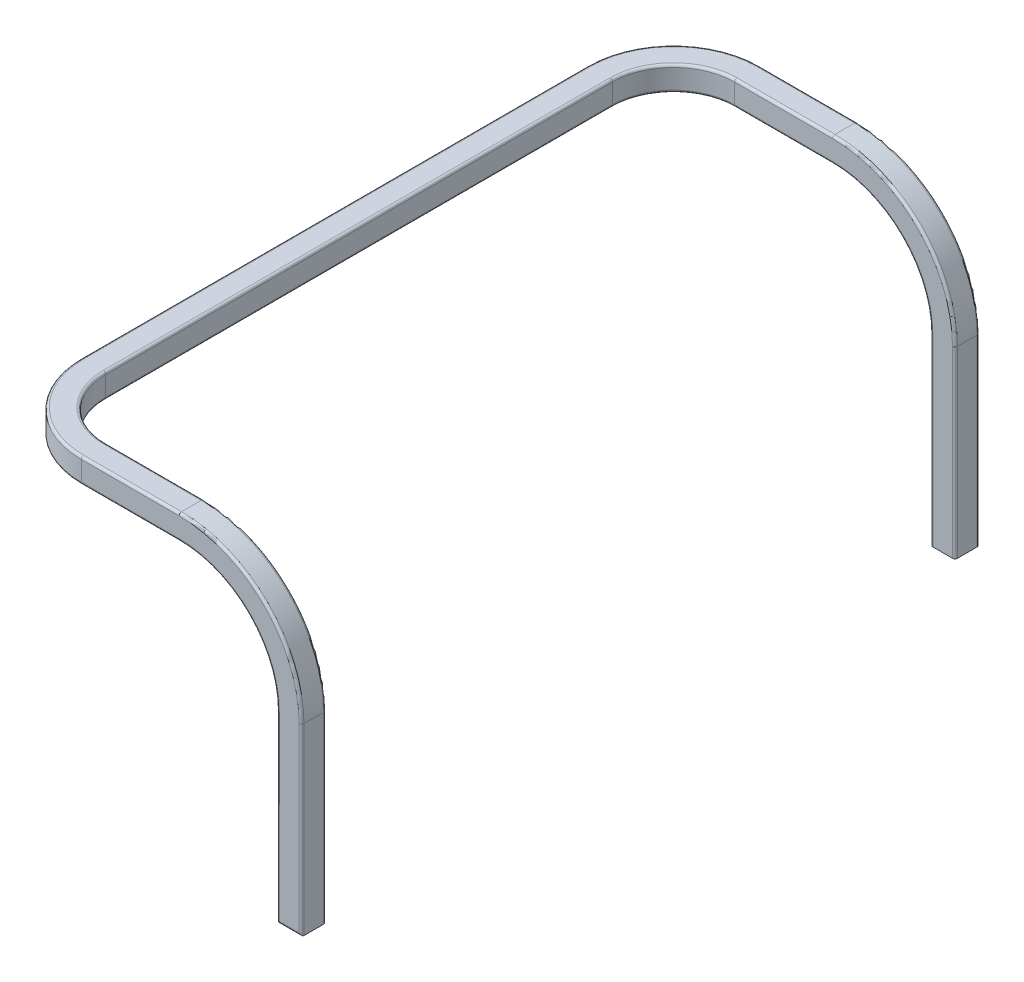
from build123d import *

# Parameters (mm, degrees)
BOSS_EXTRUDE1_DEPTH = 554
SKETCH2_W           = 357.128489267
SKETCH2_H           = 514
CUT_EXTRUDE1_DEPTH  = 466
FILLET1_R           = 50
FILLET2_R           = 70
FILLET3_R           = 2


with BuildPart() as part:
    # Sketch1 → Boss-Extrude1 (new body)
    with BuildSketch(Plane.XY):
        with BuildLine():
            Line((0, 0), (0, 150))
            ThreePointArc((0, 150), (-23.431457505, 206.568542495), (-80, 230))
            Line((-80, 230), (-230, 230))
            Line((-230, 230), (-230, 250))
            Line((-230, 250), (-80, 250))
            ThreePointArc((-80, 250), (-9.289321881, 220.710678119), (20, 150))
            Line((20, 150), (20, 0))
            Line((20, 0), (0, 0))
        make_face()
    extrude(amount=BOSS_EXTRUDE1_DEPTH)

    # Sketch2 → Cut-Extrude1 (cut)
    with BuildSketch(Plane(origin=(0, 250, 0), x_dir=(1, 0, 0), z_dir=(0, 1, 0))):
        with Locations((-31.435755366, -277)):
            Rectangle(SKETCH2_W, SKETCH2_H)
    extrude(amount=-CUT_EXTRUDE1_DEPTH, mode=Mode.SUBTRACT)

    # Fillet1
    fillet1_edges = [part.edges().sort_by_distance(p)[0] for p in [
        (-210, 240, 534),
        (-210, 240, 20),
    ]]
    fillet(fillet1_edges, radius=FILLET1_R)

    # Fillet2
    fillet2_edges = [part.edges().sort_by_distance(p)[0] for p in [
        (-230, 240, 554),
        (-230, 240, 0),
    ]]
    fillet(fillet2_edges, radius=FILLET2_R)

    # Fillet3
    fillet3_edges = [part.edges().sort_by_distance(p)[0] for p in [
        (-9.289321881, 220.710678119, 554),
        (20, 75, 0),
        (-120, 250, 554),
        (-23.431457505, 206.568542495, 554),
        (0, 75, 554),
        (0, 75, 534),
        (0, 75, 20),
        (-9.289321881, 220.710678119, 20),
        (20, 75, 20),
        (-23.431457505, 206.568542495, 20),
        (-120, 230, 20),
        (20, 75, 534),
        (-9.289321881, 220.710678119, 534),
        (-23.431457505, 206.568542495, 534),
        (10, 0, 534),
        (10, 0, 554),
        (-120, 250, 20),
        (-210, 250, 277),
        (-210, 230, 277),
        (-120, 230, 534),
        (-120, 250, 534),
        (-195.355339059, 250, 34.644660941),
        (-195.355339059, 230, 34.644660941),
        (-195.355339059, 250, 519.355339059),
        (-195.355339059, 230, 519.355339059),
        (-230, 230, 277),
        (-230, 250, 277),
        (20, 75, 554),
        (-120, 230, 554),
        (-120, 230, 0),
        (-209.497474683, 230, 533.497474683),
        (-209.497474683, 230, 20.502525317),
        (-209.497474683, 250, 533.497474683),
        (-209.497474683, 250, 20.502525317),
        (0, 75, 0),
        (-23.431457505, 206.568542495, 0),
        (-120, 250, 0),
        (-9.289321881, 220.710678119, 0),
    ]]
    fillet(fillet3_edges, radius=FILLET3_R)


solid = part.part
